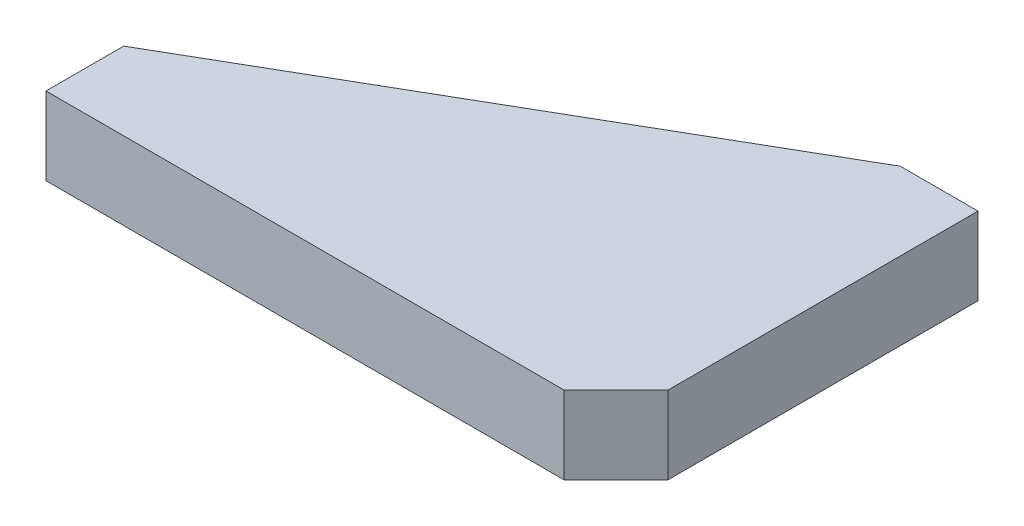
SolidWorks part; units mm, degrees
ref_plane "前视基准面" through (0, 0, 0) normal (0, 0, 1) x (1, 0, 0)
ref_plane "上视基准面" through (0, 0, 0) normal (0, 1, 0) x (1, 0, 0)
ref_plane "右视基准面" through (0, 0, 0) normal (1, 0, 0) x (0, 0, -1)
sketch "草图1" plane through (0, 0, 0) normal (0, 1, 0) x (1, 0, 0)
  line L0 (0, 0) -> (-30, 0)
  line L1 (-30, 0) -> (-220, -109.6966)
  line L2 (-220, -109.6966) -> (-220, -139.6966)
  line L3 (-220, -139.6966) -> (-20, -139.6966)
  line L4 (-20, -139.6966) -> (0, -119.6966)
  line L5 (0, -119.6966) -> (0, 0)
  dimension "D1" = 30
  dimension "D2" = 30
  dimension "D3" = 30
  dimension "D4" = 220
  dimension "D5" = 45
  dimension "D6" = 20
extrude "凸台-拉伸1" add sketch "草图1" along normal blind 30
